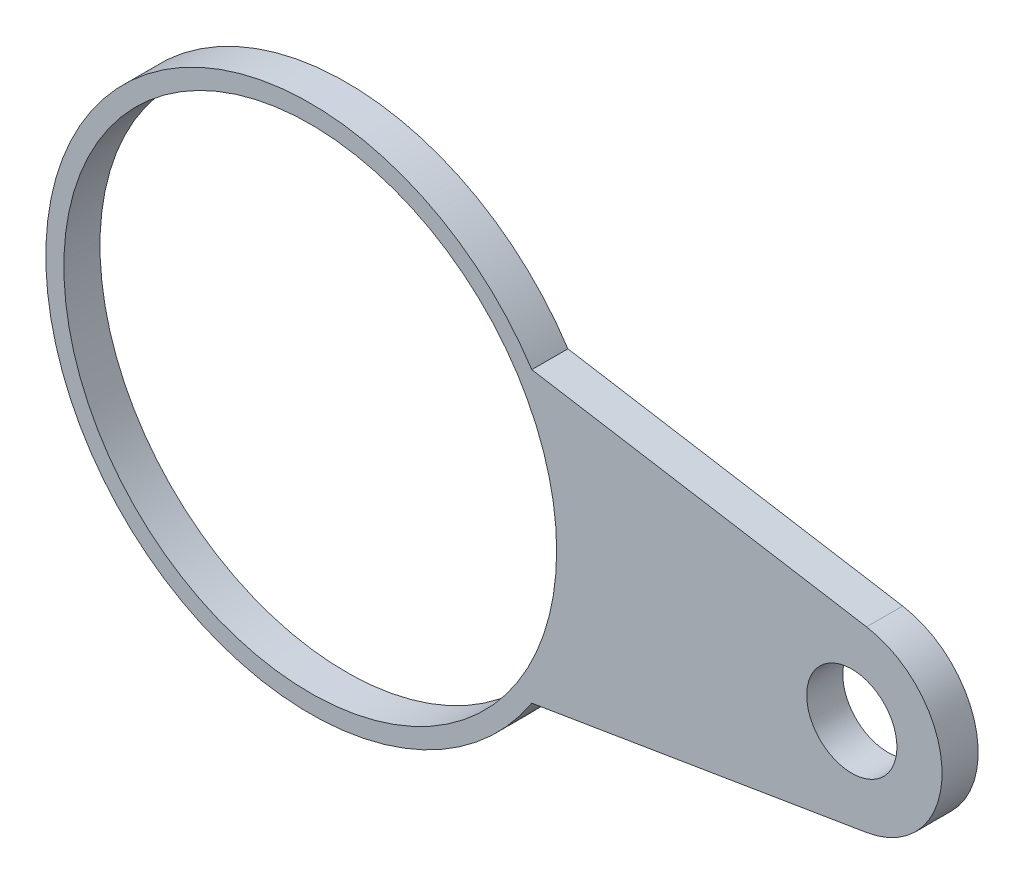
from build123d import *

# Parameters (mm, degrees)
SKETCH1_R           = 25
SKETCH1_R_2         = 136.5
BOSS_EXTRUDE1_DEPTH = 20


with BuildPart() as part:
    # Sketch1 → Boss-Extrude1 (new body)
    with BuildSketch(Plane.XY):
        with BuildLine():
            Line((122.728358581, 80), (308.159136141, 49.329793203))
            ThreePointArc((308.159136141, 49.329793203), (350, 0), (308.159136141, -49.329793203))
            Line((308.159136141, -49.329793203), (122.728358581, -80))
            ThreePointArc((122.728358581, -80), (-146.5, 0), (122.728358581, 80))
        make_face()
        with Locations((300, 0)):
            Circle(SKETCH1_R, mode=Mode.SUBTRACT)
        Circle(SKETCH1_R_2, mode=Mode.SUBTRACT)
    extrude(amount=BOSS_EXTRUDE1_DEPTH)


solid = part.part
